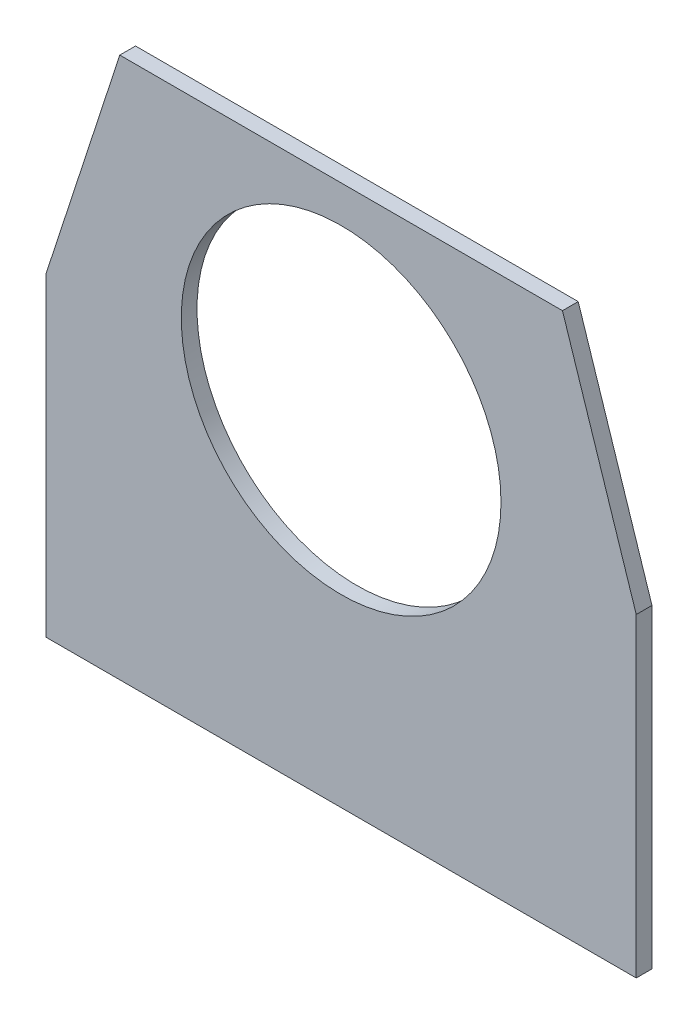
SolidWorks part; units mm, degrees
material "Q235B"
ref_plane "Front Plane" through (0, 0, 0) normal (0, 0, 1) x (1, 0, 0)
ref_plane "Top Plane" through (0, 0, 0) normal (0, 1, 0) x (1, 0, 0)
ref_plane "Right Plane" through (0, 0, 0) normal (1, 0, 0) x (0, 0, -1)
sketch "Sketch1" plane through (0, 0, 0) normal (0, 0, 1) x (1, 0, 0)
  line L0 (0, 0) -> (0, 550) construction
  line L1 (-225, 550) -> (225, 550)
  line L2 (225, 550) -> (300, 320)
  line L3 (300, 320) -> (300, 0)
  line L4 (300, 0) -> (-300, 0)
  line L5 (-300, 320) -> (-300, 0)
  line L6 (-225, 550) -> (-300, 320)
  circle A0 centre (0, 350) radius 162.5
  dimension "D1" = 325
  dimension "D2" = 550
  dimension "D3" = 350
  dimension "D4" = 600
  dimension "D5" = 450
  dimension "D6" = 320
extrude "Boss-Extrude1" add sketch "Sketch1" along normal mid plane 16
